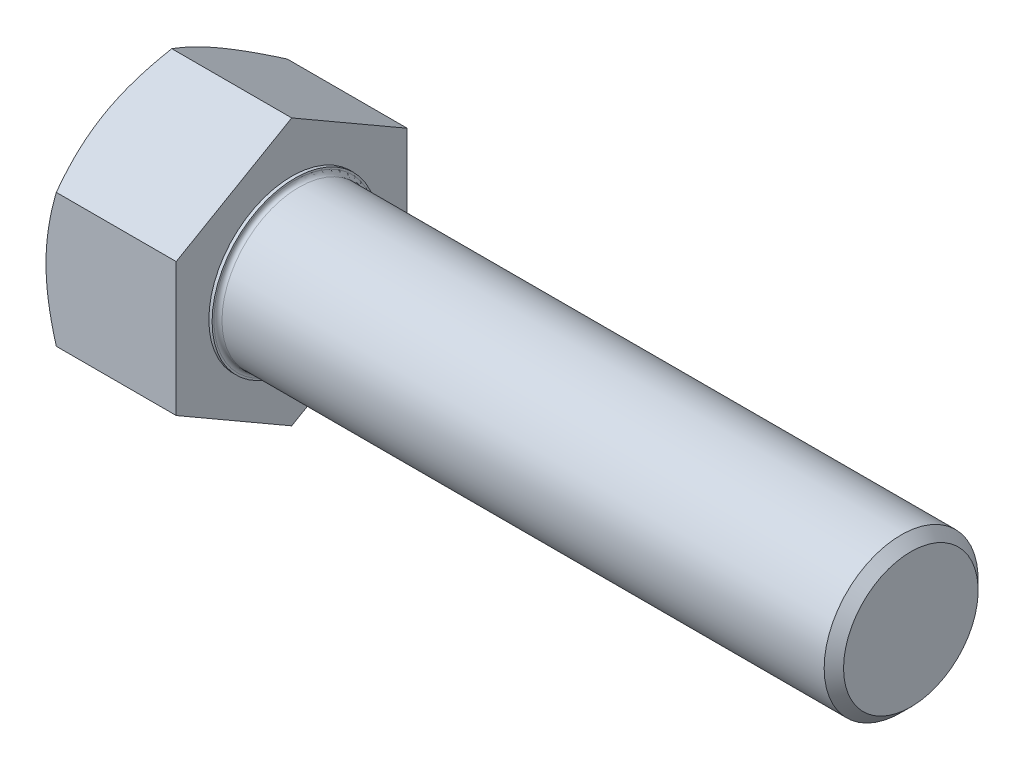
from build123d import *

# Parameters (mm, degrees)
BASE_EXTRUDE_DEPTH = 33.02
SKETCH4_W          = 0.8
SKETCH4_H          = 22.495567884
CHAMFER_2_SIZE     = 2.4
FILLET_2_R         = 1


with BuildPart() as part:
    # Sketch1 → Base-Extrude (new body)
    with BuildSketch(Plane(origin=(0, 0, 0), x_dir=(0, 0, -1), z_dir=(1, 0, 0))):
        Polygon((28.575, 16.497783942), (28.575, -16.497783942), (0, -32.995567884), (-28.575, -16.497783942), (-28.575, 16.497783942), (0, 32.995567884), align=None)
    extrude(amount=BASE_EXTRUDE_DEPTH)

    # Sketch2 → Boss-Revolve1 (revolve)
    with BuildSketch(Plane.XY, mode=Mode.PRIVATE) as boss_revolve1_sk:
        Polygon((0, 0), (185.42, 0), (185.42, 13.8), (185.42, 19.05), (27.8072, 19.05), (0, 19.05), align=None)
    revolve(boss_revolve1_sk.sketch.rotate(Axis((0, 0, 0), (1, 0, 0)), 90), axis=Axis((0, 0, 0), (1, 0, 0)))

    # Sketch3 → Cut-Revolve1 (revolve, cut)
    with BuildSketch(Plane.XY):
        Polygon((0, 28.575), (5.438967404, 37.995567884), (5.438967404, 42.995567884), (-10, 42.995567884), (-10, 28.575), align=None)
    revolve(axis=Axis((0, 0, 0), (1, 0, 0)), mode=Mode.SUBTRACT)

    # Sketch4 → Cut-Revolve3 (revolve, cut)
    with BuildSketch(Plane.XY, mode=Mode.PRIVATE) as cut_revolve3_sk:
        with Locations((32.62, 31.747783942)):
            Rectangle(SKETCH4_W, SKETCH4_H)
    revolve(cut_revolve3_sk.sketch.rotate(Axis((0, 0, 0), (1, 0, 0)), 90), axis=Axis((0, 0, 0), (1, 0, 0)), mode=Mode.SUBTRACT)

    # Chamfer 2
    chamfer_2_edges = [part.edges().sort_by_distance(p)[0] for p in [
        (185.42, 0, -19.05),
    ]]
    chamfer(chamfer_2_edges, length=CHAMFER_2_SIZE)

    # Fillet 2
    fillet_2_edges = [part.edges().sort_by_distance(p)[0] for p in [
        (33.02, 0, -19.05),
    ]]
    fillet(fillet_2_edges, radius=FILLET_2_R)


solid = part.part
